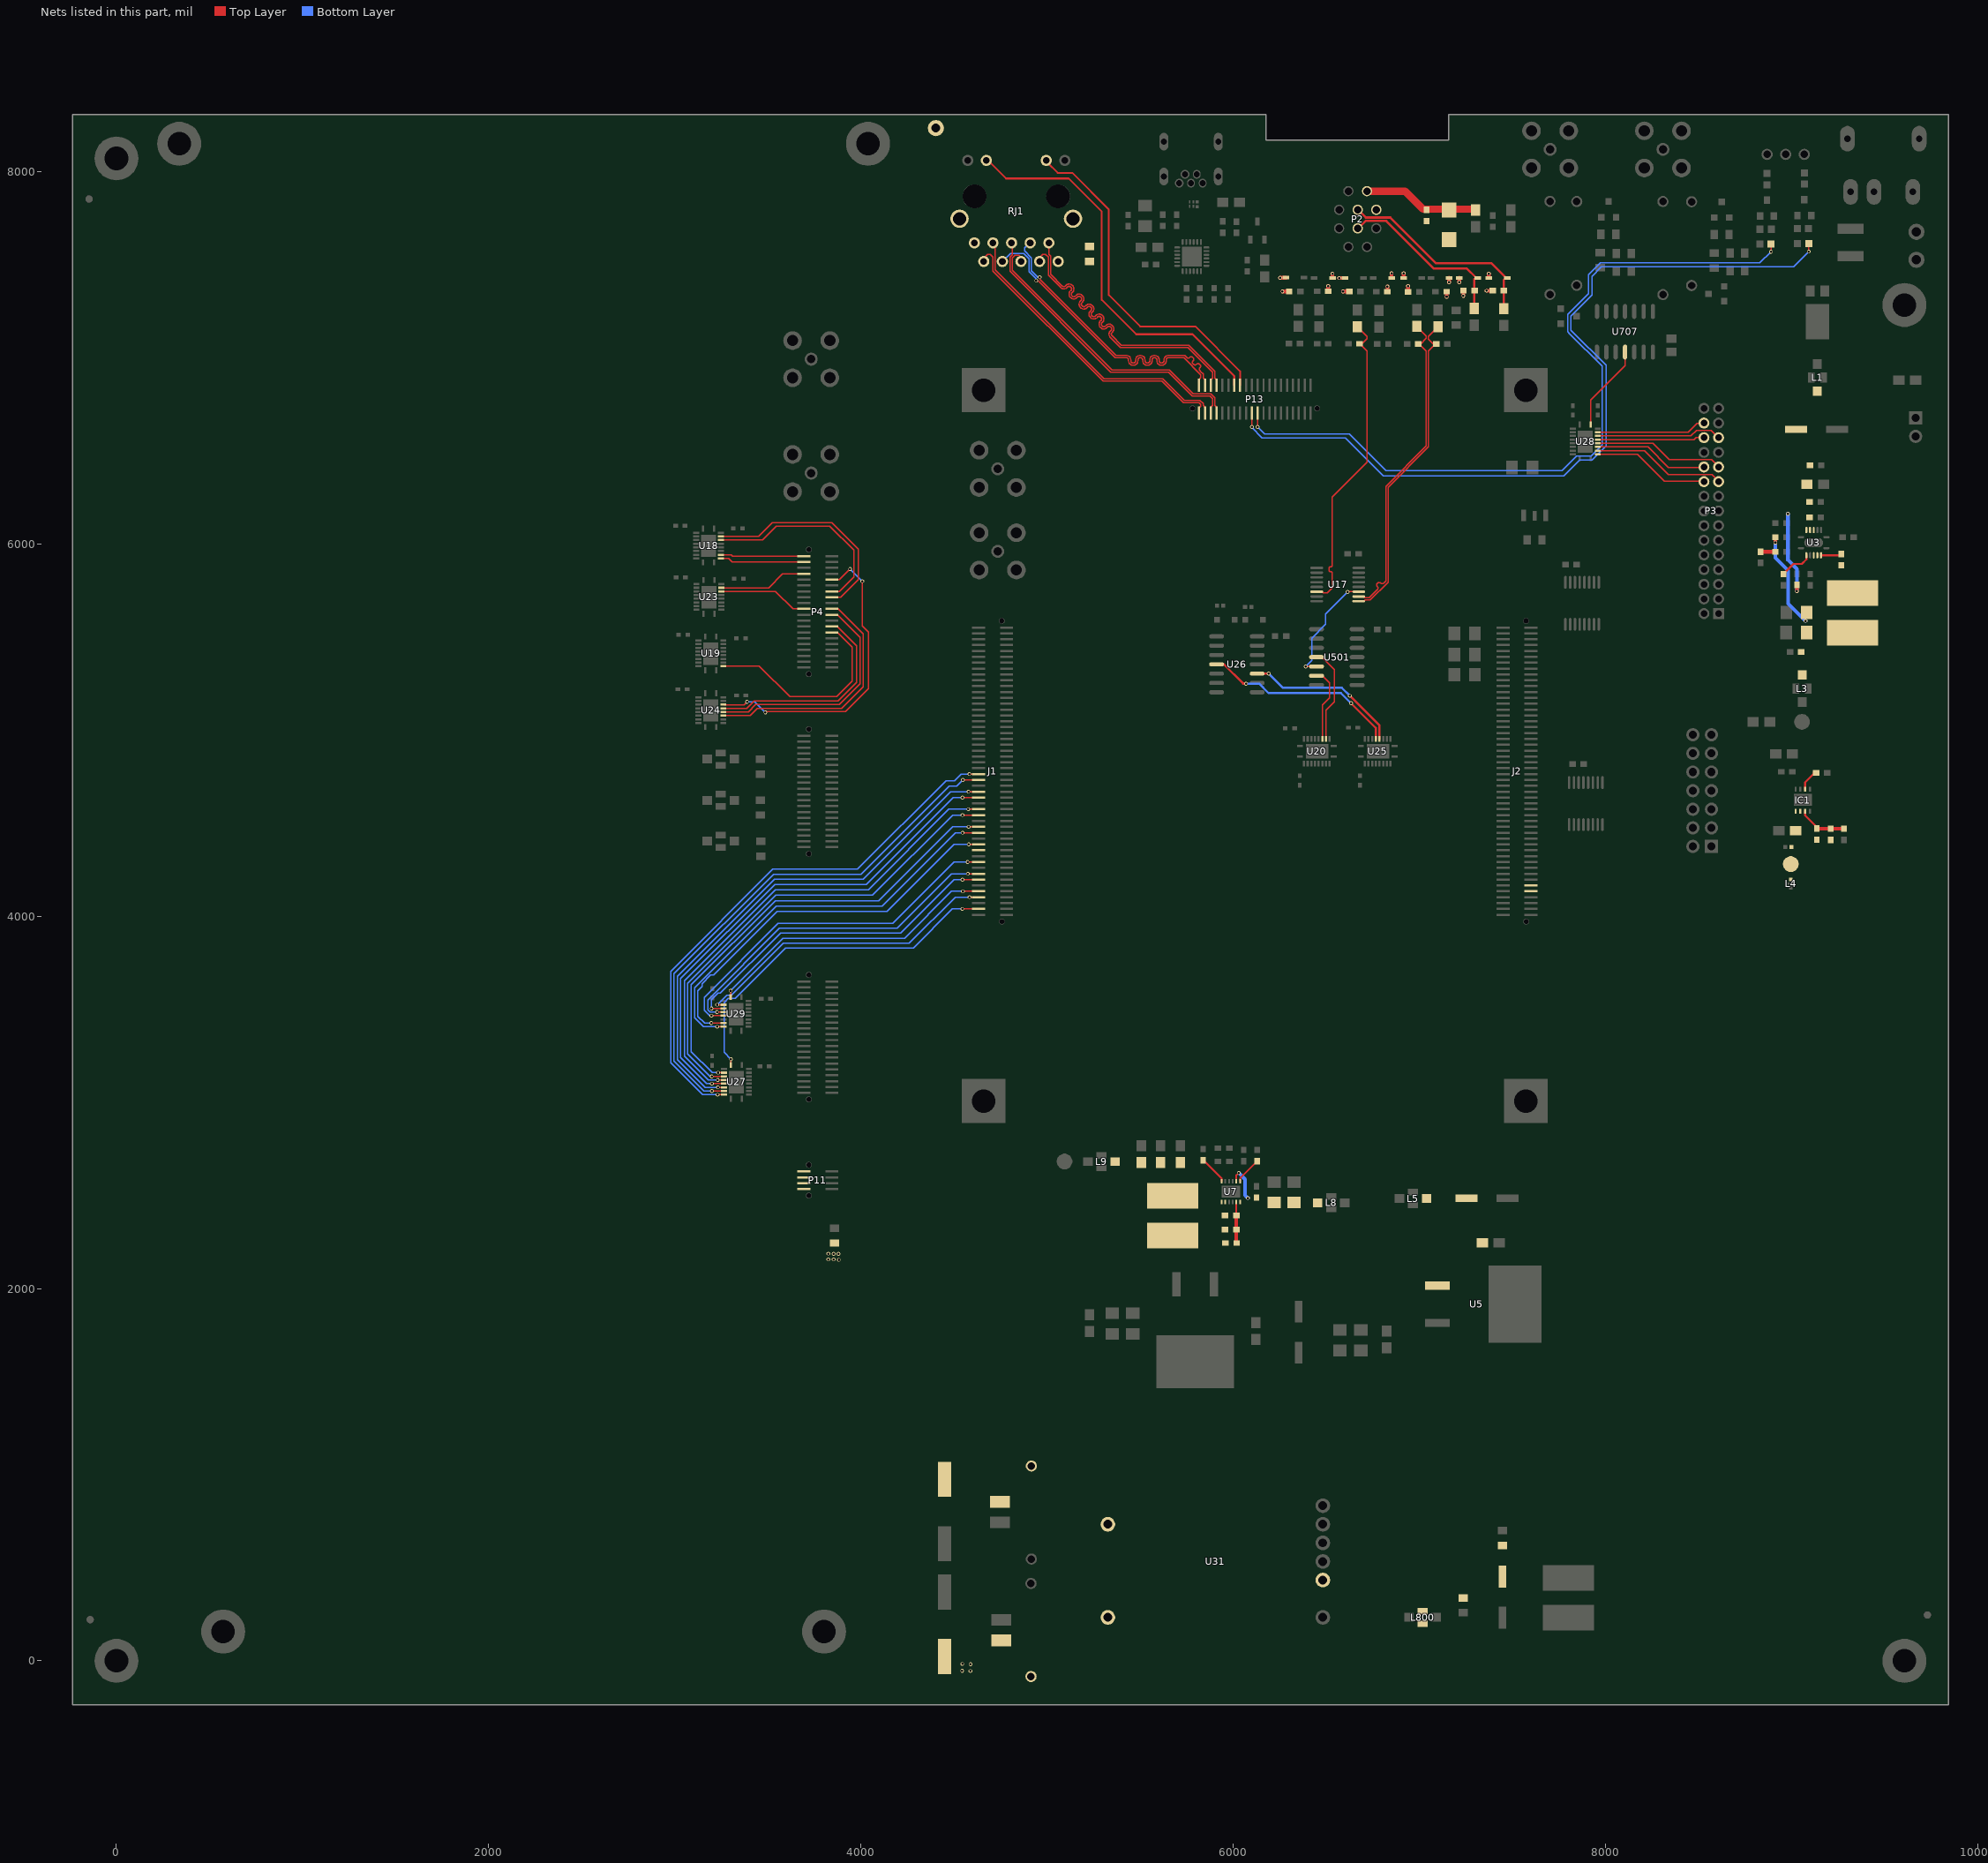
[diagram p0: the nets of this part, all layers, seen from the top]
# Altium PCB MISC82191.PcbDoc (part 7 of 9)
Units mil, origin at the board's own origin, x right, y up, seen from the top; angles counter-clockwise.
Board outline 10078.74 x 8543.31 mil, 4 copper layers (Top Layer, GND, POWER, Bottom Layer); 238 components, 299 nets, 1297 pads, 1665 vias.

## Via types
v1: diameter 20, hole 12, Top Layer to Bottom Layer, 1664 vias
v2: diameter 40, hole 20, Top Layer to Bottom Layer, 1 vias

## Nets (pads, with @x,y where several pads share a name; then routed paths per layer and width w, separated by ;. In a path a pad name is that pad's centre, name@x,y a point inside that pad or via, vN(x,y) a via of type N, cw(c..) or ccw(c..) an arc to the next point about the centre after c; other vN are vias at no path point) (continued)
"ENCODER B_P": C59.1 L15.1 U17.6 | length 1654
  Top Layer w6: U17.6@6448.78,5743.2 6476.74,5743.2 6483.53,5736.4 6505.05,5736.4 6532.78,5764.13 6532.78,5838.16 6532.78,5842.06 ccw(c6523.68,5842.06) 6523.68,5851.16 6523.11,5851.16 cw(c6523.11,5860.26) 6514.01,5860.26 6514.01,5868.06 cw(c6523.11,5868.06) 6523.11,5877.16 6523.68,5877.16 ccw(c6523.68,5886.26) 6532.78,5886.26 6532.78,5896.16 6532.78,6252.13 6719.78,6439.13 6719.78,7037.16 6681.78,7075.16 C59.1@6678.78,7075.16 ; L15.1@6667.78,7166.16 6719.78,7114.16 6719.78,7102.16 C59.1@6690.78,7073.16
"ENCODER BB": U20.13 U501.4 | length 487.3
  Top Layer w6: U501.4@6474.78,5393.16 6543.78,5324.16 6543.78,5151.16 6498.57,5105.94 U20.13@6498.57,4953.18
"ENCODER Z": U17.11 U501.5 | length 609.9
  Top Layer w6: v1(6389.21,5341.72) U501.5@6447.66,5341.72 ; v1@6616.82,5743.2 U17.11@6674.43,5743.2
  Bottom Layer w6: v1(6389.21,5341.72) 6421.78,5374.29 6421.78,5494.16 6495.78,5568.16 6495.78,5623.16 v1(6614.78,5742.16)
"ENCODER Z_N": C68（NC）.1 L18.1 U17.9 | length 1707.8
  Top Layer w6: U17.9@6674.43,5692.02 6701.64,5692.02 6708.43,5698.81 6735.43,5698.81 6831.78,5795.16 6831.78,6304.16 7048.78,6521.16 7048.78,7037.16 C68（NC）.1@7080.78,7069.16 ; C68（NC）.1@7078.78,7069.16 7048.78,7099.16 7048.78,7115.16 L18.1@7099.78,7166.16
"ENCODER Z_P": C66.1 L17.1 U17.10 | length 1708.8
  Top Layer w6: U17.10@6674.43,5717.61 6700.33,5717.61 6707.12,5710.81 6730.46,5710.81 6773.29,5753.64 6774.21,5754.56 ccw(c6765.94,5762.84) 6774.21,5771.11 cw(c6782.49,5779.38) 6774.21,5787.65 6776.05,5789.49 cw(c6784.33,5781.22) 6792.6,5789.49 ccw(c6800.87,5797.77) 6809.14,5789.49 6819.78,5800.13 6819.78,6309.13 7036.78,6526.13 7036.78,7037.16 C66.1@7008.78,7065.16 ; L17.1@6985.78,7168.16 7036.78,7117.16 7036.78,7104.16 C66.1@7004.78,7072.16
"ENCODER ZZ": U20.14 U501.6 | length 365.6
  Top Layer w6: U20.14@6478.88,4953.18 6478.88,5134.26 6517.78,5173.16 6517.78,5253.16 U501.6@6482.78,5288.16
ETH_LED1: P13.16 RJ1.12 | length 1840.8
  Top Layer w10: RJ1.12@5003.78,8046.16 5056.78,7993.16 5134.78,7993.16 5331.78,7796.16 5331.78,7337.16 5500.78,7168.16 5796.78,7168.16 6037.14,6927.8 P13.16@6037.14,6852.42
ETH_LED2: P13.14 RJ1.13 | length 2124.3
  Top Layer w10: RJ1.13@4686.78,8056.16 4779.78,7963.16 5115.78,7963.16 5293.78,7785.16 5293.78,7311.16 5478.78,7126.16 5781.78,7126.16 6005.65,6902.29 P13.14@6005.65,6852.42
ETH_TD0_N: P13.6 RJ1.3 | length 1603.9
  Top Layer w6: RJ1.3@4959.78,7517.16 4959.78,7538.16 4976.78,7555.16 4991.78,7555.16 5006.78,7540.16 5006.78,7443.16 5073.62,7376.31 ccw(c5089.96,7392.65) 5106.29,7376.31 5110.39,7380.42 cw(c5118.24,7372.57) 5126.09,7380.42 5128.78,7377.73 cw(c5120.93,7369.88) 5132.03,7369.88 cw(c5120.93,7369.88) 5128.78,7362.03 5124.68,7357.93 ccw(c5141.01,7341.59) 5124.68,7325.26 5127.36,7322.57 ccw(c5143.7,7338.91) 5160.03,7322.57 5164.13,7326.68 cw(c5171.98,7318.83) 5179.83,7326.68 5182.52,7323.99 cw(c5174.67,7316.14) 5185.77,7316.14 cw(c5174.67,7316.14) 5182.52,7308.29 5178.42,7304.19 ccw(c5194.75,7287.85) 5178.42,7271.52 5181.1,7268.83 ccw(c5197.44,7285.17) 5213.77,7268.83 5217.87,7272.93 cw(c5225.72,7265.09) 5233.57,7272.93 5236.26,7270.25 cw(c5228.41,7262.4) 5239.51,7262.4 cw(c5228.41,7262.4) 5236.26,7254.55 5232.16,7250.45 ccw(c5248.49,7234.11) 5232.16,7217.78 5234.84,7215.09 ccw(c5251.18,7231.43) 5267.51,7215.09 5271.61,7219.19 cw(c5279.46,7211.35) 5287.31,7219.19 5290,7216.51 cw(c5282.15,7208.66) 5293.25,7208.66 cw(c5282.15,7208.66) 5290,7200.81 5285.9,7196.71 ccw(c5302.23,7180.37) 5285.9,7164.04 5288.58,7161.35 ccw(c5304.92,7177.69) 5321.25,7161.35 5325.35,7165.45 cw(c5333.2,7157.61) 5341.05,7165.45 5343.74,7162.77 cw(c5335.89,7154.92) 5346.99,7154.92 cw(c5335.89,7154.92) 5343.74,7147.07 5339.64,7142.97 ccw(c5355.97,7126.63) 5339.64,7110.3 5393.78,7056.16 5755.81,7056.16 5889.41,6922.56 5889.41,6890.79 5879.66,6881.04 P13.6@5879.66,6852.42
ETH_TD0_P: P13.8 RJ1.2 | length 1604.1
  Top Layer w6: RJ1.2@5009.43,7617.16 5008.78,7616.51 5008.78,7555.13 5018.78,7545.13 5018.78,7448.13 5082.11,7384.8 ccw(c5089.96,7392.65) 5097.81,7384.8 5101.91,7388.9 cw(c5118.24,7372.57) 5134.58,7388.9 5137.26,7386.21 cw(c5120.93,7369.88) 5144.03,7369.88 cw(c5120.93,7369.88) 5137.26,7353.55 5133.16,7349.44 ccw(c5141.01,7341.59) 5133.16,7333.75 5135.85,7331.06 ccw(c5143.7,7338.91) 5151.55,7331.06 5155.65,7335.16 cw(c5171.98,7318.83) 5188.32,7335.16 5191,7332.47 cw(c5174.67,7316.14) 5197.77,7316.14 cw(c5174.67,7316.14) 5191,7299.81 5186.9,7295.7 ccw(c5194.75,7287.85) 5186.9,7280.01 5189.59,7277.32 ccw(c5197.44,7285.17) 5205.29,7277.32 5209.39,7281.42 cw(c5225.72,7265.09) 5242.06,7281.42 5244.74,7278.73 cw(c5228.41,7262.4) 5251.51,7262.4 cw(c5228.41,7262.4) 5244.74,7246.06 5240.64,7241.96 ccw(c5248.49,7234.11) 5240.64,7226.27 5243.33,7223.58 ccw(c5251.18,7231.43) 5259.03,7223.58 5263.13,7227.68 cw(c5279.46,7211.35) 5295.8,7227.68 5298.48,7224.99 cw(c5282.15,7208.66) 5305.25,7208.66 cw(c5282.15,7208.66) 5298.48,7192.32 5294.38,7188.22 ccw(c5302.23,7180.37) 5294.38,7172.53 5297.07,7169.84 ccw(c5304.92,7177.69) 5312.77,7169.84 5316.87,7173.94 cw(c5333.2,7157.61) 5349.54,7173.94 5352.22,7171.25 cw(c5335.89,7154.92) 5358.99,7154.92 cw(c5335.89,7154.92) 5352.22,7138.58 5348.12,7134.48 ccw(c5355.97,7126.63) 5348.12,7118.79 5398.75,7068.16 5760.78,7068.16 5901.41,6927.53 5901.41,6891.53 5911.16,6881.78 P13.8@5911.16,6852.42
ETH_TD1_N: P13.2 RJ1.7 | length 1597.7
  Top Layer w6: v1@4951.71,7414.22 4956.78,7409.16 5365.81,7000.16 5426.68,7000.16 cw(c5426.68,6989.06) 5437.78,6989.06 5437.78,6983.26 ccw(c5460.88,6983.26) 5460.88,6960.16 5464.68,6960.16 ccw(c5464.68,6983.26) 5487.78,6983.26 5487.78,6989.06 cw(c5498.88,6989.06) 5498.88,7000.16 5502.68,7000.16 cw(c5502.68,6989.06) 5513.78,6989.06 5513.78,6983.26 ccw(c5536.88,6983.26) 5536.88,6960.16 5540.68,6960.16 ccw(c5540.68,6983.26) 5563.78,6983.26 5563.78,6989.06 cw(c5574.88,6989.06) 5574.88,7000.16 5578.68,7000.16 cw(c5578.68,6989.06) 5589.78,6989.06 5589.78,6983.26 ccw(c5612.88,6983.26) 5612.88,6960.16 5616.68,6960.16 ccw(c5616.68,6983.26) 5639.78,6983.26 5639.78,6989.06 cw(c5650.88,6989.06) 5650.88,7000.16 5734.4,7000.16 5826.42,6908.14 5826.42,6897.78 ; P13.2@5816.67,6852.42 5816.67,6883.05 5826.42,6892.8 5826.42,6897.55
  Bottom Layer w6: RJ1.7@4761.78,7519.78 4802.78,7560.78 4874.78,7560.78 4903.78,7531.78 4903.78,7462.19 4940.78,7425.19 v1@4940.78,7416.16
  other v1: 4941.84,7414.22
ETH_TD1_P: P13.4 RJ1.4 | length 1597
  Top Layer w6: 4960.84,7422.09 5370.78,7012.16 5426.68,7012.16 cw(c5426.68,6989.06) 5449.78,6989.06 5449.78,6983.26 ccw(c5460.88,6983.26) 5460.88,6972.16 5464.68,6972.16 ccw(c5464.68,6983.26) 5475.78,6983.26 5475.78,6989.06 cw(c5498.88,6989.06) 5498.88,7012.16 5502.68,7012.16 cw(c5502.68,6989.06) 5525.78,6989.06 5525.78,6983.26 ccw(c5536.88,6983.26) 5536.88,6972.16 5540.68,6972.16 ccw(c5540.68,6983.26) 5551.78,6983.26 5551.78,6989.06 cw(c5574.88,6989.06) 5574.88,7012.16 5578.68,7012.16 cw(c5578.68,6989.06) 5601.78,6989.06 5601.78,6983.26 ccw(c5612.88,6983.26) 5612.88,6972.16 5616.68,6972.16 ccw(c5616.68,6983.26) 5627.78,6983.26 5627.78,6989.06 cw(c5650.88,6989.06) 5650.88,7012.16 5739.37,7012.16 5748.76,7002.76 5750.6,7000.93 ccw(c5757.96,7008.28) 5765.31,7000.93 5766.81,7002.43 cw(c5774.17,6995.08) 5781.52,7002.43 5785.2,6998.75 cw(c5777.85,6991.4) 5785.2,6984.04 5783.7,6982.54 ccw(c5791.05,6975.19) 5783.7,6967.83 5787.37,6964.16 ccw(c5794.73,6971.51) 5802.08,6964.16 5803.58,6965.66 cw(c5810.94,6958.31) 5818.29,6965.66 5821.97,6961.98 cw(c5814.61,6954.63) 5821.97,6947.28 5820.47,6945.77 ccw(c5827.82,6938.42) 5820.47,6931.06 5826.26,6925.26 5838.42,6913.11 5838.42,6901.78 ; 5838.42,6902.52 5838.42,6901.78 ; P13.4@5848.17,6852.42 5848.17,6882.77 5838.42,6892.52 5838.42,6901.78
  Bottom Layer w6: RJ1.4@4900.78,7612.78 4878.78,7590.78 4878.78,7573.75 4915.78,7536.75 4915.78,7467.16 4949.78,7433.16 v1@4959.78,7433.16 ; RJ1.4@4909.78,7611.16 RJ1.4@4914.78,7616.16
  other v1: 4960.23,7432.61
ETH_TD2_N: P13.5 RJ1.6 | length 1602.5
  Top Layer w6: RJ1.6@4819.29,7606.64 4813.78,7601.13 4813.78,7553.13 4800.78,7540.13 4800.78,7465.16 5342.78,6923.16 5651.81,6923.16 5780.81,6794.16 5874.78,6794.16 5889.41,6779.53 5889.41,6743.79 5879.66,6734.04 P13.5@5879.66,6702.82
ETH_TD2_P: P13.7 RJ1.5 | length 1602.1
  Top Layer w6: RJ1.5@4859.78,7518.16 4859.78,7539.16 4848.78,7550.16 4827.78,7550.16 4812.78,7535.16 4812.78,7470.13 5347.75,6935.16 5656.78,6935.16 5785.78,6806.16 5879.75,6806.16 5901.41,6784.5 5901.41,6744.53 5911.16,6734.78 P13.7@5911.16,6702.82
ETH_TD3_N: P13.1 RJ1.9 | length 1607.6
  Top Layer w6: RJ1.9@4663.78,7527.16 4663.78,7538.16 4679.78,7554.16 4695.78,7554.16 4708.78,7541.16 4708.78,7466.19 5300.81,6874.16 5616.81,6874.16 5732.81,6758.16 5816.81,6758.16 5826.42,6748.55 5826.42,6739.8 5816.67,6730.05 P13.1@5816.67,6702.82
ETH_TD3_P: P13.3 RJ1.8 | length 1607.1
  Top Layer w6: RJ1.8@4714.78,7606.16 4720.78,7600.16 4720.78,7471.16 5305.78,6886.16 5621.78,6886.16 5737.78,6770.16 5821.78,6770.16 5838.42,6753.52 5838.42,6743.52 5848.17,6733.77 P13.3@5848.17,6702.82
GATE/ON: U28.20 U707.11 | length 451.3
  Top Layer w6: U28.20@7920.78,6649.16 7920.78,6772.16 8105.78,6957.16 U707.11@8105.78,7023.78
HGND: C100.2 C101.2 C102.2 C103.2 L800.2 L800.4 R44.1 RZ1.1 RZ2.1 U31.4 U31.6
  other v1: 4587.78,-54.59 4543.78,-53.59 4588.78,-17.59 4544.78,-16.59 3880.78,2154.41 3824.78,2156.41 3852.78,2156.41 3852.78,2186.41 3879.78,2186.41 3824.78,2187.41
"HP FILT EN": P4.3 U18.12 | length 560.9
  Top Layer w6: U18.12@3248.14,5922.33 U18.12@3255.78,5922.33 ; U18.12@3255.78,5922.16 3289.78,5922.16 3309.17,5902.76 P4.3@3694.21,5902.76 3587.39,5902.76
HT: C98.1 C99.1 P11.1 P11.3 P11.5 P11.7 R43.2 U31.7
HV_SCL: J2.A46
HV_SDA: J2.A45
IN1: P4.19 U23.17 | length 482.9
  Top Layer w6: U23.17@3250.24,5744.76 3540.18,5744.76 3634.14,5650.8 P4.19@3694.21,5650.8
IN2: P4.7 U23.18 | length 572.2
  Top Layer w6: U23.18@3250.24,5764.44 3504.06,5764.44 3579.39,5839.77 P4.7@3694.21,5839.77 3597.17,5839.77
"IN ZERO A": U25.16 U26.4 | length 1057.1
  Top Layer w12: U26.4@5910.78,5353.16 5950.78,5353.16 6053.78,5250.16 v1@6070.78,5250.16 ; v1(6633.78,5144.16) 6766.51,5011.43 U25.16@6766.51,4953.18
  Bottom Layer w12: v1(6068.78,5249.16) 6139.78,5249.16 6189.78,5199.16 6578.78,5199.16 v1(6633.78,5144.16)
"IN ZERO B": U25.15 U26.10 | length 844.3
  Top Layer w12: U26.10@6128.82,5303.16 v1(6190.78,5303.16) ; v1(6626.78,5184.16) 6786.2,5024.74 U25.15@6786.2,4953.18
  Bottom Layer w12: v1(6190.78,5303.16) 6266.78,5227.16 6583.78,5227.16 v1(6626.78,5184.16)
IO20: P3.28 U28.18 | length 583.3
  Top Layer w6: U28.18@7958.24,6599.82 8445.19,6599.82 8492.78,6647.41 P3.28@8521.78,6647.41
IO21: P3.25 U28.17 | length 664.9
  Top Layer w6: U28.17@7958.24,6580.13 8459.5,6580.13 8488.56,6609.19 8569,6609.19 P3.25@8598.78,6579.41
IO22: P3.26 U28.16 | length 570.5
  Top Layer w6: U28.16@7958.24,6560.45 8474.82,6560.45 8486.78,6572.41 P3.26@8523.78,6572.41
IO23: P3.21 U28.15 | length 701.1
  Top Layer w6: U28.15@7958.24,6540.76 8254.43,6540.76 8341.8,6453.39 8570.8,6453.39 P3.21@8607.78,6416.41
IO24: P3.22 U28.14 | length 630
  Top Layer w6: U28.14@7958.24,6521.08 8229.11,6521.08 8338.78,6411.41 8472.78,6411.41 ; 8489.78,6411.41 8472.78,6411.41 ; P3.22@8525.78,6411.41 8472.78,6411.41
IO25: P3.19 U28.13 | length 740.3
  Top Layer w6: U28.13@7958.24,6501.39 8069.78,6501.39 ; 8102.54,6501.39 8069.78,6501.39 ; P3.19@8600.78,6344.41 8572.22,6372.97 8337.22,6372.97 8208.8,6501.39 8069.78,6501.39
IO26: P3.20 U28.12 | length 659.5
  Top Layer w6: U28.12@7958.24,6481.71 8020.78,6481.71 ; 8026.23,6481.71 8020.78,6481.71 ; 8490.51,6337.41 8464.78,6337.41 ; P3.20@8526.78,6337.41 8464.78,6337.41 ; 8020.78,6481.71 8171.48,6481.71 8315.78,6337.41 8464.78,6337.41
K0: P4.10 U24.17 | length 1664.2
  Top Layer w6: U24.17@3264.78,5135.78 3371.78,5135.78 v1(3387.78,5151.78) ; v1(3486.4,5094.78) 3490.78,5099.16 3917.16,5099.16 4040.78,5222.78 4040.78,5525.78 4007.16,5559.4 v1(4007.16,5799.78) ; P4.10@3843.82,5808.28 3884.9,5808.28 v1(3941.78,5865.16)
  Bottom Layer w6: v1(3387.78,5151.78) 3429.4,5151.78 v1(3486.4,5094.78) ; v1(3941.78,5865.16) v1(4007.16,5799.78)
K1: J1.B26 U27.9 | length 2945.9
  Top Layer w6: v1(3229.95,3041.33) U27.9@3264.38,3041.33 ; v1(4582.23,4763.61) J1.B26@4632.75,4763.61
  Bottom Layer w6: v1(3229.95,3041.33) 3149.61,3041.33 2977.78,3213.16 2977.78,3704.16 3526.03,4252.41 3981.78,4252.41 4457.78,4728.41 4502.78,4728.41 4537.53,4763.16 v1@4585.78,4763.16
K2: J1.B27 U27.8 | length 2877.3
  Top Layer w6: v1(3198.92,3061.02) U27.8@3264.38,3061.02 ; v1(4547.83,4732.11) J1.B27@4632.75,4732.11
  Bottom Layer w6: v1(3198.92,3061.02) 3155.92,3061.02 2995.78,3221.16 2995.78,3691.16 3530.03,4225.41 4000.78,4225.41 4473.78,4698.41 4514.13,4698.41 v1(4547.83,4732.11) ; v1@4546.78,4731.16 v1@4549.78,4734.16
K3: J1.B33 U27.4 | length 2566.3
  Top Layer w6: v1(3198.38,3139.76) U27.4@3264.38,3139.76 ; v1(4545.76,4543.13) J1.B33@4632.75,4543.13
  Bottom Layer w6: v1(3198.38,3139.76) 3189.18,3139.76 3069.78,3259.16 3069.78,3640.16 3543.03,4113.41 4062.78,4113.41 4492.5,4543.13 v1(4545.76,4543.13) ; v1@4544.78,4543.16 v1@4547.78,4546.16
K4: J1.B29 U27.7 | length 2793.3
  Top Layer w6: v1(3231.24,3080.7) U27.7@3264.38,3080.7 ; v1(4577.82,4669.12) J1.B29@4632.75,4669.12
  Bottom Layer w6: v1(3231.24,3080.7) 3163.24,3080.7 3013.78,3230.16 3013.78,3677.16 3536.03,4199.41 4012.78,4199.41 4482.49,4669.12 v1(4577.82,4669.12) ; v1@4577.82,4670.16 v1@4581.78,4670.16
K5: J1.B32 U27.5 | length 2638.4
  Top Layer w6: v1(3230.87,3120.07) U27.5@3264.38,3120.07 ; v1(4577.25,4574.63) J1.B32@4632.75,4574.63
  Bottom Layer w6: v1(3230.87,3120.07) 3180.87,3120.07 3052.78,3248.16 3052.78,3654.16 3541.03,4142.41 4040.78,4142.41 4473,4574.63 v1(4577.25,4574.63) ; v1@4577.25,4575.16 v1@4583.78,4575.16
K6: J1.B35 U27.3 | length 2488.8
  Top Layer w6: v1(3232.5,3159.44) U27.3@3264.38,3159.44 ; v1(4578.76,4480.14) J1.B35@4632.75,4480.14
  Bottom Layer w6: v1(3232.5,3159.44) 3200.5,3159.44 3087.78,3272.16 3087.78,3631.16 3539.91,4083.28 4095.65,4083.28 4492.51,4480.14 v1(4578.76,4480.14) ; v1@4580.78,4482.16 v1(4578.76,4480.14) ; v1@4585.78,4480.16 v1(4578.76,4480.14)
K7: J1.B49 U27.1 | length 1932.8
  Top Layer w6: U27.1@3301.78,3200.78 v1(3301.78,3232.16) ; v1(4544.82,4039.2) J1.B49@4632.75,4039.2
  Bottom Layer w6: v1(3301.78,3232.16) 3264.78,3269.16 3264.78,3536.16 3287.78,3559.16 3324.78,3559.16 3594.91,3829.28 4281.65,3829.28 4491.57,4039.2 v1(4544.82,4039.2) ; v1@4544.82,4040.16 4547.78,4040.16 v1@4549.78,4042.16
K8: J1.B36 U29.9 | length 2215.9
  Top Layer w6: v1(3226.95,3406.33) U29.9@3262.38,3406.33 ; v1(4546.27,4448.65) J1.B36@4632.75,4448.65
  Bottom Layer w6: v1(3226.95,3406.33) 3153.61,3406.33 3105.78,3454.16 3105.78,3616.16 3545.03,4055.41 4114.78,4055.41 4508.02,4448.65 v1(4546.27,4448.65) ; v1@4545.78,4448.16 v1(4546.27,4448.65) ; v1@4549.78,4452.16 v1(4546.27,4448.65)
K9: J1.B38 U29.8 | length 2142.8
  Top Layer w6: v1(3195.92,3426.02) U29.8@3262.38,3426.02 ; v1(4579.28,4385.65) J1.B38@4632.75,4385.65
  Bottom Layer w6: v1(3195.92,3426.02) 3159.92,3426.02 3123.78,3462.16 3123.78,3600.16 3145.78,3622.16 3145.78,3637.16 3192.78,3684.16 3207.78,3684.16 ; 3208.78,3684.16 3207.78,3684.16 ; v1@4580.78,4387.16 v1@4579.78,4386.16 ; v1@4584.78,4386.16 v1@4579.78,4386.16 ; 3207.78,3684.16 3549.91,4026.28 4139.65,4026.28 4499.53,4386.16 v1@4579.78,4386.16
K10: J1.B44 U29.4 | length 1816.8
  Top Layer w6: v1(3197.38,3504.76) U29.4@3262.38,3504.76 ; v1(4545.26,4196.68) J1.B44@4632.75,4196.68
  Bottom Layer w6: v1(3197.38,3504.76) 3197.38,3550.63 3232.91,3586.16 3243.78,3586.16 3568.03,3910.41 4213.78,3910.41 4500.05,4196.68 v1(4545.26,4196.68) ; v1@4545.26,4197.16 4546.78,4197.16 v1@4547.78,4198.16
K11: J1.B47 U29.3 | length 1681.3
  Top Layer w6: v1(3227.06,3524.44) U29.3@3262.38,3524.44 ; v1(4583.75,4102.19) J1.B47@4632.75,4102.19
  Bottom Layer w6: v1(3227.06,3524.44) 3278.78,3576.16 3303.78,3576.16 3581.91,3854.28 4259.65,3854.28 4507.56,4102.19 v1(4583.75,4102.19) ; v1@4583.75,4104.16 v1@4584.78,4104.16
K12: J1.B41 U29.6 | length 1964.6
  Top Layer w6: v1(3196.55,3465.39) U29.6@3262.38,3465.39 ; v1(4572.79,4291.16) J1.B41@4632.75,4291.16
  Bottom Layer w6: v1(3196.55,3465.39) 3186.55,3465.39 3157.78,3494.16 3157.78,3564.16 3555.03,3961.41 4170.78,3961.41 4500.53,4291.16 v1@4574.78,4291.16
K13: J1.B43 U29.5 | length 1881.3
  Top Layer w6: v1(3226.87,3485.07) U29.5@3262.38,3485.07 ; v1(4574.76,4228.17) J1.B43@4632.75,4228.17
  Bottom Layer w6: v1(3226.87,3485.07) 3188.87,3485.07 3176.78,3497.16 3176.78,3550.16 3562.41,3935.78 4194.15,3935.78 4486.53,4228.16 4572.78,4228.16 v1@4574.78,4230.16
K14: J1.B30 U27.6 | length 2724.9
  Top Layer w6: v1(3199.01,3100.39) U27.6@3264.38,3100.39 ; v1(4545.24,4637.62) J1.B30@4632.75,4637.62
  Bottom Layer w6: v1(3199.01,3100.39) 3171.55,3100.39 3031.78,3240.16 3031.78,3665.16 3538.03,4171.41 4029.78,4171.41 4495.99,4637.62 v1(4545.24,4637.62) ; v1@4543.78,4639.16 v1@4547.78,4635.16
K15: J1.B39
K16: J1.B46 U29.1 | length 1594.6
  Top Layer w6: U29.1@3299.78,3565.78 v1(3299.78,3600.16) ; v1(4547.31,4133.68) J1.B46@4632.75,4133.68
  Bottom Layer w6: v1(3299.78,3600.16) 3299.78,3601.16 3580.91,3882.28 4233.65,3882.28 4485.05,4133.68 v1(4547.31,4133.68) ; v1@4545.78,4135.16 v1(4547.31,4133.68) ; v1(4547.31,4133.68) v1(4547.31,4133.68) ; v1@4549.78,4131.16 v1(4547.31,4133.68)
KGND: C51.2 C52.2 C53.2 C56.2 C57.2 C58.2 C62.1 C63(NC).1 C64.1 C65.1 P2.3 pad.1@4402.78,8233.78 RJ1.10 RJ1.15 RJ1.16 U8.1 U9.1 U10.1 U11.1 U12.1 U13.2 U14.2 U15.2 U16.2 | length 449.3
  Top Layer w20: v1(6251.78,7430.16) U11.1@6282.57,7430.16 ; v1(6264.78,7356.16) C57.2@6300.78,7356.16 ; C58.2@6510.78,7357.16 v1(6510.78,7385.16) ; U12.1@6532.99,7429.16 v1(6532.99,7451.94) ; v1(6569.78,7428.16) U8.1@6601.57,7428.16 ; v1(6589.78,7356.16) C52.2@6623.78,7356.16 ; C65.1@6828.78,7355.16 v1(6828.78,7383.16) ; U16.2@6850.99,7428.16 v1(6850.99,7453.94) ; U15.2@6915.57,7429.16 v1(6915.57,7453.94) ; C64.1@6939.78,7354.16 v1(6939.78,7385.16) ; v1(7146.78,7327.16) 7146.78,7355.16 ; v1(7159.99,7406.37) U14.2@7159.99,7429.16 ; v1(7214.57,7406.37) U10.1@7214.57,7429.16 ; v1(7236.78,7332.16) C56.2@7236.78,7360.16 ; v1(7361.78,7360.16) C53.2@7393.78,7360.16 ; U9.1@7373.57,7429.16 v1(7373.57,7451.94)
LB_A0: P4.28 U19.12 | length 1121.9
  Top Layer w6: U19.12@3260.24,5343.33 3453.61,5343.33 3617.78,5179.16 3870.78,5179.16 3953.78,5262.16 3953.78,5445.16 3874.13,5524.81 P4.28@3843.82,5524.81
LB_A1: P4.26 U24.16 | length 1144.8
  Top Layer w6: U24.16@3260.24,5117.07 3385.69,5117.07 3425.78,5157.16 3876.78,5157.16 3975.78,5256.16 3975.78,5453.16 3872.63,5556.31 P4.26@3843.82,5556.31
LB_A2: P4.22 U24.15 | length 1249.5
  Top Layer w6: U24.15@3260.24,5097.39 3395.01,5097.39 3434.78,5137.16 3884.78,5137.16 3995.78,5248.16 3995.78,5497.16 3873.64,5619.3 P4.22@3843.82,5619.3
LB_A4: P4.20 U24.14 | length 1323.8
  Top Layer w6: U24.14@3260.24,5077.7 3404.32,5077.7 3442.78,5116.16 3896.78,5116.16 4011.78,5231.16 4011.78,5516.16 3877.14,5650.8 P4.20@3843.82,5650.8
LB_A5: P4.16 U18.18 | length 1170.6
  Top Layer w6: U18.18@3248.14,6040.44 3450.06,6040.44 3523.78,6114.16 3842.78,6114.16 3984.78,5972.16 3984.78,5807.16 3891.41,5713.79 P4.16@3843.82,5713.79
LB_A6: P4.14 U18.17 | length 1091.1
  Top Layer w6: U18.17@3248.14,6020.76 3471.38,6020.76 3545.78,6095.16 3832.78,6095.16 3961.78,5966.16 3961.78,5823.16 3883.91,5745.28 P4.14@3843.82,5745.28
LED1: P13.19 R25.1 | length 4449.7
  Top Layer w6: v1(6100.13,6628.05) P13.19@6100.13,6702.82 ; v1@9092.4,7576.03 R25.1@9092.4,7613.09
  Bottom Layer w6: v1(6100.13,6628.05) 6100.13,6625.05 6155.78,6569.41 6603.78,6569.41 6807.78,6365.41 7775.78,6365.41 7861.78,6451.41 7926.78,6451.41 8002.78,6527.41 8002.78,6959.41 7823.78,7138.41 ; 7821.78,7140.41 7823.78,7138.41 ; v1(9092.78,7570.41) 9010.78,7488.41 7978.78,7488.41 7927.78,7437.41 7927.78,7337.41 7814.78,7224.41 7814.78,7147.41 7823.78,7138.41
LED2: P13.21 R26.1 | length 4194.3
  Top Layer w6: v1(6131.63,6628.26) P13.21@6131.63,6702.82 ; v1(8889.4,7569.03) R26.1@8889.4,7611.09
  Bottom Layer w6: v1(6131.63,6628.26) 6168.48,6591.41 6623.78,6591.41 6821.78,6393.41 7766.78,6393.41 7845.78,6472.41 7922.78,6472.41 7965.78,6515.41 7981.78,6531.41 7981.78,6954.41 7806.78,7129.41 ; 7803.78,7132.41 7806.78,7129.41 ; v1(8889.4,7569.03) 8829.78,7509.41 7972.78,7509.41 7908.78,7445.41 7908.78,7344.41 7796.78,7232.41 7796.78,7139.41 7806.78,7129.41
"LP FILT EN": P4.1 U18.13 | length 449.3
  Top Layer w6: U18.13@3248.14,5942.02 U18.13@3251.78,5942.02 ; U18.13@3251.78,5942.16 3302.78,5942.16 3310.68,5934.26 P4.1@3694.21,5934.26
NetC7_2: C7.2 IC1.6 | length 123.7
  Top Layer w11: IC1.6@9072.96,4681.31 9072.96,4719.34 C7.2@9125.78,4772.16 ; C7.2@9119.78,4773.16 C7.2@9130.78,4773.16
NetC8_1: C8.1 C9.1 C10.1 C15.1 C16.1 L1.3 R2.1 U3.4 U3.5 U3.6 | length 467.9
  Top Layer w20: v1(9028.78,5746.16) R2.1@9028.78,5779.16
  Bottom Layer w20: v1(8980.78,6161.16) 8980.78,5913.16 9028.78,5865.16 v1(9028.78,5746.16)
NetC11_1: C11.1 U3.13 | length 107.1
  Top Layer w11: U3.13@9158.24,5938.72 C11.1@9265.34,5938.72
NetC11_2: C11.2 L2.2 U3.11 U3.12
NetC12_1: C12.1 IC1.3 R1.2 R3.1 | length 254.6
  Top Layer w11: IC1.3@9072.96,4563.16 9072.96,4541.98 R3.1@9134.78,4480.16
  Top Layer w20: R3.1@9134.78,4470.16 C12.1@9209.78,4470.16 R1.2@9280.78,4470.16
NetC12_2: C12.2 C13.2 C14.2 IC1.1 IC1.2 L4.1 R3.2 TP2.1
NetC17_1: C17.1 C18.1 C19.1 L2.1 L3.1 R4.2 | length 517.1
  Top Layer w20: v1(8912.78,6007.16) R4.2@8912.78,6036.16
  Bottom Layer w20: v1(8912.78,6007.16) 8912.78,5926.16 8981.78,5857.16 8981.78,5679.16 v1(9074.78,5586.16)
NetC20_1: C20.1 U3.9 | length 162.6
  Top Layer w11: C20.1@8966.78,5849.16 9009.78,5892.16 9054.78,5892.16 9079.5,5916.88 U3.9@9079.5,5938.72
NetC21_1: C21.1 R9.2 | length 77
  Top Layer w20: C21.1@8831.78,5957.16 R9.2@8908.78,5957.16
NetC23_1: C23.1 C24.2 L5.3 U5.1
NetC40_2: C40.2 U7.1 | length 133.8
  Top Layer w10: U7.1@6036.59,2575.83 6036.59,2591.97 C40.2@6119.78,2675.16
NetC41_1: C41.1 C42.1 C43.1 L8.1 U7.2 U7.12 | length 206
  Top Layer w10: U7.2@6016.91,2575.83 6016.91,2608.29 v1(6029.78,2621.16)
  Bottom Layer w20: v1(6029.78,2621.16) 6063.78,2587.16 6063.78,2501.16 v1(6078.78,2486.16)
NetC44_1: C44.1 C45.1 C46.1 L10.2 U7.8
NetC44_2: C44.2 C45.2 C46.2 U7.11 | length 211
  Top Layer w10: C46.2@6016.91,2401.03 U7.11@6016.91,2465.59
  Top Layer w20: C44.2@6016.59,2246.35 C45.2@6016.59,2316.83 C46.2@6016.59,2392.83
NetC47_2: C47.2 C48.2 C49.2 L9.1 L10.1 U7.7
NetC50_1: C50.1 U7.6 | length 148
  Top Layer w10: C50.1@5844.78,2685.16 5938.17,2591.77 U7.6@5938.17,2575.83
NetC51_1: C51.1 RJ1.1
NetC53_1: C53.1 L11.2 P2.10 U9.2 | length 1109.7
  Top Layer w12: P2.10@6675.78,7790.16 6712.78,7753.16 6843.78,7753.16 7089.78,7507.16 7387.78,7507.16 7464.78,7430.16 7464.78,7429.16 7453.78,7418.16 C53.1@7453.78,7360.16 L11.2@7453.78,7263.16
NetC56_1: C56.1 L12.2 P2.9 U10.2 | length 948.6
  Top Layer w6: P2.9@6668.78,7697.16 P2.9@6672.78,7701.16
  Top Layer w12: P2.9@6674.78,7699.16 6710.78,7735.16 6822.78,7735.16 7078.78,7479.16 7255.78,7479.16 7302.78,7432.16 7305.78,7432.16 7294.78,7421.16 L12.2@7294.78,7265.16
NetC62_2: C62.2 L19.2 P2.4 U13.1 | length 623.2
  Top Layer w40: P2.4@6718.78,7895.16 6922.78,7895.16 7019.78,7798.16 L19.2@7301.78,7798.16